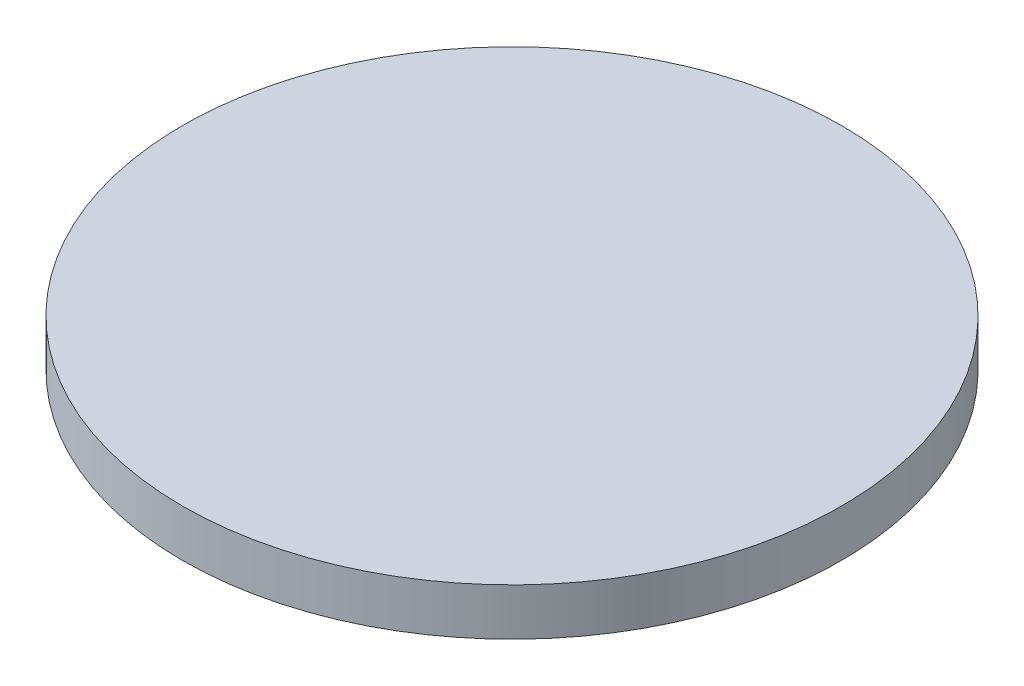
from build123d import *

# Parameters (mm, degrees)
SKETCH1_R           = 14
BOSS_EXTRUDE1_DEPTH = 2


with BuildPart() as part:
    # Sketch1 → Boss-Extrude1 (new body)
    with BuildSketch(Plane(origin=(0, 0, 0), x_dir=(1, 0, 0), z_dir=(0, 1, 0))):
        with Locations(Location((0, 0, 0), (0, 0, 270))):
            Circle(SKETCH1_R)
    extrude(amount=BOSS_EXTRUDE1_DEPTH)


solid = part.part
